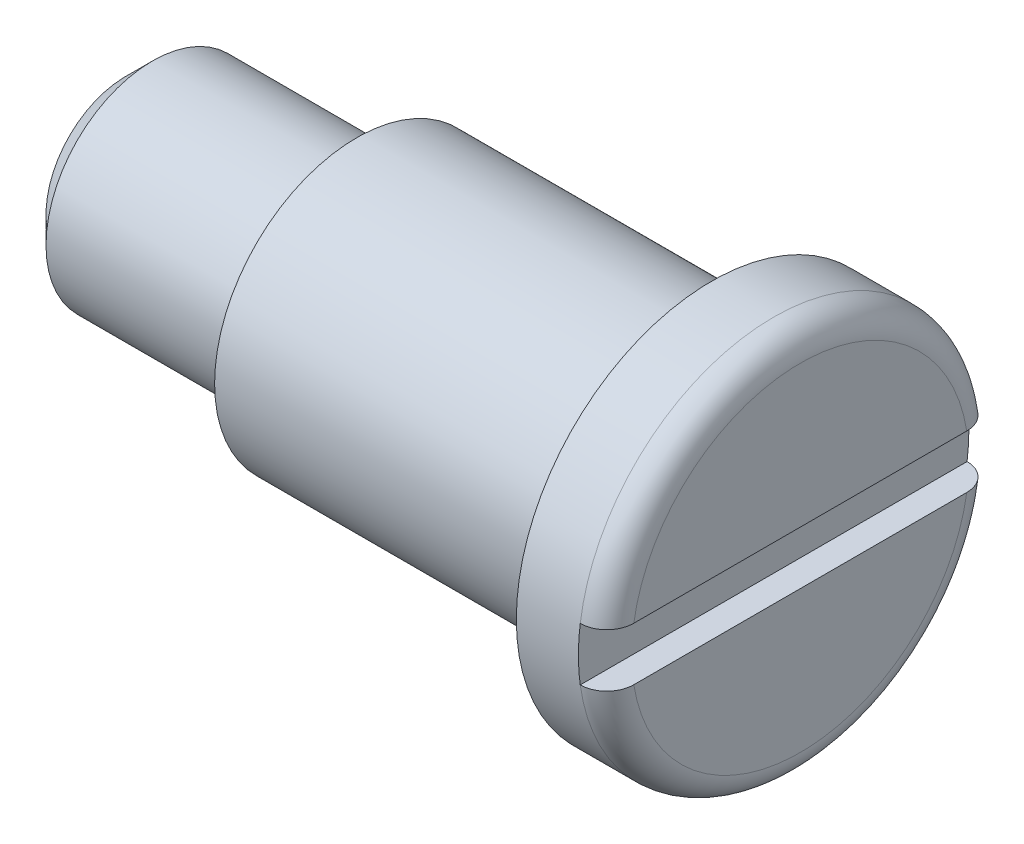
SolidWorks part; units mm, degrees
ref_plane "Front Plane" through (0, 0, 0) normal (0, 0, 1) x (1, 0, 0)
ref_plane "Top Plane" through (0, 0, 0) normal (0, 1, 0) x (1, 0, 0)
ref_plane "Right Plane" through (0, 0, 0) normal (1, 0, 0) x (0, 0, -1)
sketch "Sketch1" plane through (0, 0, 0) normal (0, 1, 0) x (1, 0, 0)
  line L0 (-19, 0) -> (19, 0) construction
  line L1 (-19, 0) -> (-19, 6)
  line L2 (-19, 6) -> (-6, 6)
  line L3 (-6, 6) -> (-6, 8)
  line L4 (-6, 8) -> (14, 8)
  line L5 (14, 8) -> (14, 11)
  line L6 (14, 11) -> (19, 11)
  line L7 (19, 11) -> (19, 0)
  line L8 (-19, 0) -> (19, 0)
  dimension "D1" = 19
  dimension "D2" = 38
  dimension "D3" = 5
  dimension "D4" = 20
  dimension "D5" = 6
  dimension "D6" = 2
  dimension "D7" = 11
revolve "Revolve1" add sketch "Sketch1" angle 360 about L0
sketch "Sketch2" plane through (19, 0, 0) normal (1, 0, 0) x (0, 0, -1)
  line L2 (-12.2862, 1.5) -> (13.9926, 1.5)
  line L3 (-12.2862, 1.5) -> (-12.2862, -1.5)
  line L4 (-12.2862, -1.5) -> (13.9926, -1.5)
  line L5 (13.9926, 1.5) -> (13.9926, -1.5)
  dimension "D1" = 3
extrude "Cut-Extrude1" cut sketch "Sketch2" against normal blind 1.5
fillet "Fillet1" radius 1.5 2 edges at (19, -11, 0) (19, 11, 0)
chamfer "Chamfer1" distance 1.5 angle 45 1 edges at (-19, 0, 6)
